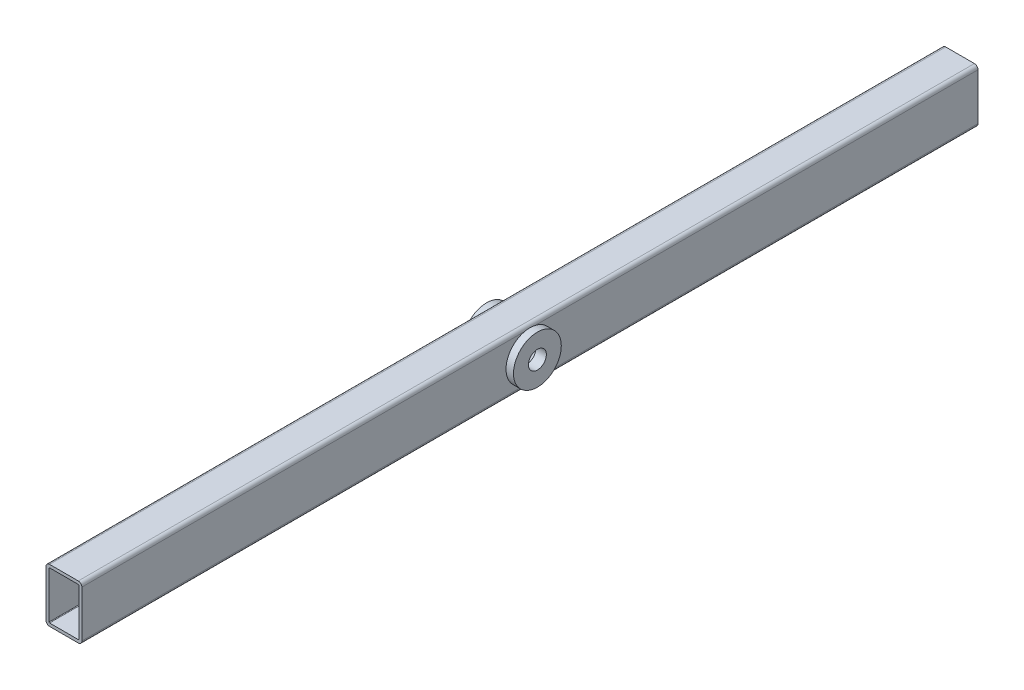
SolidWorks part; units mm, degrees
ref_plane "Front Plane" through (0, 0, 0) normal (0, 0, 1) x (1, 0, 0)
ref_plane "Top Plane" through (0, 0, 0) normal (0, 1, 0) x (1, 0, 0)
ref_plane "Right Plane" through (0, 0, 0) normal (1, 0, 0) x (0, 0, -1)
sketch "Sketch 1" plane through (0, 0, 0) normal (0, 0, 1) x (1, 0, 0)
  line L0 (0, 112.2283) -> (0, -129.0761) construction
  line L1 (-101.6304, 0) -> (92.9348, 0) construction
  line L2 (0, 90) -> (-48, 90)
  line L3 (-60, 78) -> (-60, 0)
  line L4 (0, 80) -> (-48, 80)
  line L5 (-50, 78) -> (-50, 0)
  line L6 (50, 78) -> (50, -78)
  line L7 (0, 80) -> (48, 80)
  line L8 (60, 78) -> (60, -78)
  line L9 (0, 90) -> (48, 90)
  line L10 (0, -90) -> (48, -90)
  line L11 (0, -80) -> (48, -80)
  line L12 (-50, -78) -> (-50, 0)
  line L13 (0, -80) -> (-48, -80)
  line L14 (-60, -78) -> (-60, 0)
  line L15 (0, -90) -> (-48, -90)
  arc A0 (-48, 90) -> (-60, 78) centre (-48, 78) ccw
  arc A1 (-48, 80) -> (-50, 78) centre (-48, 78) ccw
  arc A2 (48, 80) -> (50, 78) centre (48, 78) cw
  arc A3 (48, 90) -> (60, 78) centre (48, 78) cw
  arc A4 (48, -90) -> (60, -78) centre (48, -78) ccw
  arc A5 (48, -80) -> (50, -78) centre (48, -78) ccw
  arc A6 (-48, -80) -> (-50, -78) centre (-48, -78) cw
  arc A7 (-48, -90) -> (-60, -78) centre (-48, -78) cw
  point P35 (60, 0)
  point P36 (50, 0)
  dimension "D3" = 12
  dimension "D1" = 120
  dimension "D2" = 180
  dimension "D4" = 10
extrude "Boss-Extrude 1" add sketch "Sketch 1" along normal mid plane 3000
sketch "Sketch 2" plane through (0, 0, 0) normal (1, 0, 0) x (0, 0, -1)
  line L0 (-3097.5058, 0) -> (4474.3922, 0) construction
  line L1 (0, 1005.3059) -> (0, -540.6737) construction
  line L2 (-1500, -78) -> (-1500, 78) construction
  circle A1 centre (-1700, 0) radius 25 construction
  circle A2 centre (1700, 0) radius 25 construction
  circle A3 centre (0, 0) radius 30
  circle A4 centre (1700, 0) radius 100 construction
  circle A5 centre (-1700, 0) radius 100 construction
  dimension "D2" = 60
  dimension "D3" = 200
  dimension "D4" = 50
  dimension "D5" = 200
extrude "Cut-Extrude 1" cut sketch "Sketch 2" against normal through all both and the other way through all
sketch "Sketch 3" plane through (60, 0, 0) normal (1, 0, 0) x (0, 0, -1)
  circle A0 centre (0, 0) radius 80
  circle A1 centre (0, 0) radius 30 construction
  circle A2 centre (0, 0) radius 30
  dimension "D1" = 50
extrude "Boss-Extrude 2" add sketch "Sketch 3" along normal blind 25
mirror "Mirror 1" about plane through (0, 0, 0) normal (1, 0, 0) of "Boss-Extrude 2"
